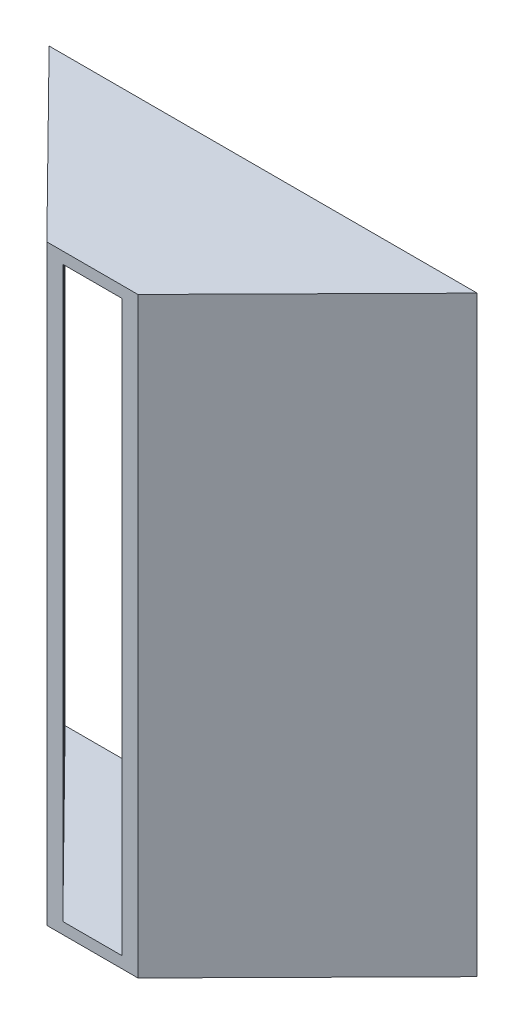
from build123d import *

# Parameters (mm, degrees)
BOSS_EXTRUDE1_DEPTH = 520
SHELL1_T            = -10


with BuildPart() as part:
    # Sketch1 → Boss-Extrude1 (new body)
    with BuildSketch(Plane(origin=(0, 0, 0), x_dir=(1, 0, 0), z_dir=(0, 1, 0))):
        Polygon((0, 0), (40, 0), (188, 150), (0, 150), align=None)
    boss_extrude1 = extrude(amount=BOSS_EXTRUDE1_DEPTH)

    # Mirror1: Boss-Extrude1 across plane
    add(boss_extrude1.mirror(Plane(origin=(0, 520, 0), x_dir=(0, 0, 1), z_dir=(1, 0, 0))))

    # Shell1
    shell1_openings = [part.faces().sort_by_distance(p)[0] for p in [
        (0, 260, -150),
        (0, 260, 0),
    ]]
    offset(amount=SHELL1_T, openings=shell1_openings, kind=Kind.INTERSECTION)


solid = part.part
